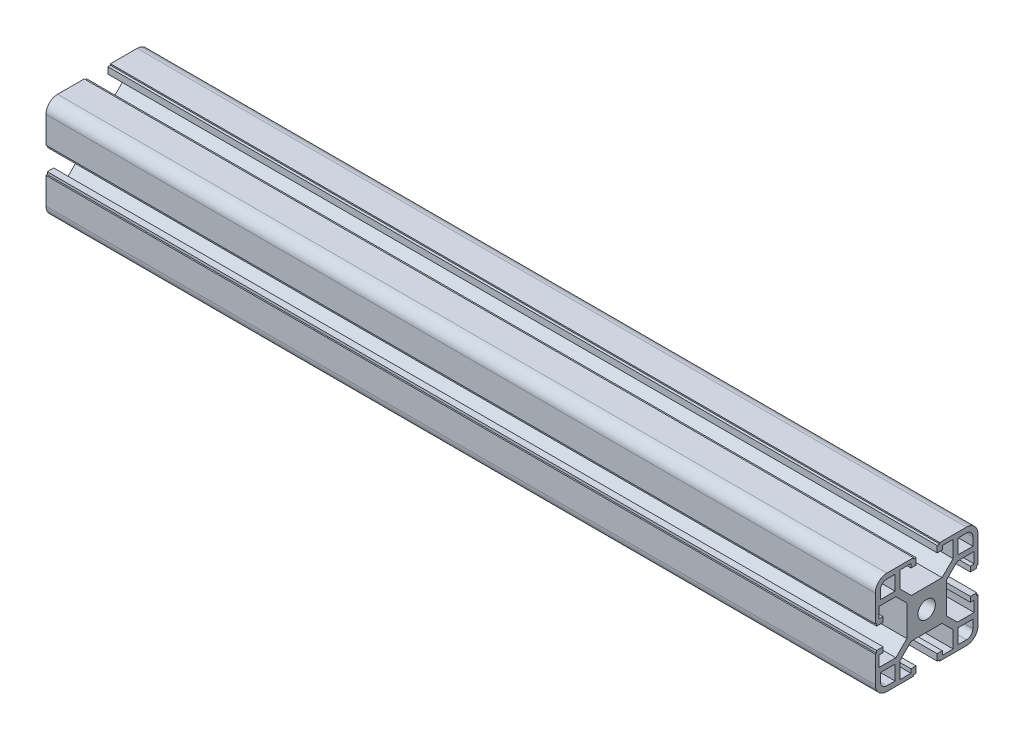
SolidWorks part; units mm, degrees
ref_plane "Front Plane" through (0, 0, 0) normal (0, 0, 1) x (1, 0, 0)
ref_plane "Top Plane" through (0, 0, 0) normal (0, 1, 0) x (1, 0, 0)
ref_plane "Right Plane" through (0, 0, 0) normal (1, 0, 0) x (0, 0, -1)
sketch "草图1" plane through (0, 0, 0) normal (0, 0, 1) x (1, 0, 0)
  line L0 (-984.975, 0) -> (-661.975, 0)
  dimension "D1" = 323
other "Aluminium profile 40 X 40B X R4.5(1)"
ref_plane "Plane1" through (-984.975, 0, 0) normal (1, 0, 0) x (0, 1, 0)
sketch "Sketch1" plane through (-984.975, 0, 0) normal (1, 0, 0) x (0, 1, 0)
  line L0 (-5.1, 20) -> (-5.1, 19.5)
  line L1 (-5.1, 19.5) -> (-4.1, 19.5)
  line L2 (-4.1, 19.5) -> (-4.1, 17)
  line L3 (-6.1, 18.5) -> (-10.3, 18.5)
  line L4 (-15.5, -20) -> (-5.1, -20)
  line L5 (-20, -15.5) -> (-20, -5.1)
  line L6 (15.5, 20) -> (5.1, 20)
  line L7 (20, 15.5) -> (20, 5.1)
  line L8 (0, 14.8756) -> (0, 0) construction
  line L9 (0, 0) -> (14.1675, 0) construction
  line L10 (-10.3, 18.5) -> (-10.3, 12)
  line L11 (-10.3, 12) -> (-6, 7.7)
  line L12 (-6, 7.7) -> (6, 7.7)
  line L13 (10.3, 12) -> (6, 7.7)
  line L14 (10.3, 18.5) -> (10.3, 12)
  line L15 (6.1, 18.5) -> (10.3, 18.5)
  line L16 (4.1, 19.5) -> (4.1, 17)
  line L17 (5.1, 19.5) -> (4.1, 19.5)
  line L18 (5.1, 20) -> (5.1, 19.5)
  line L19 (-5.1, 20) -> (-15.5, 20)
  line L20 (20, 5.1) -> (19.5, 5.1)
  line L21 (12.3, 18) -> (15.5, 18)
  line L22 (12.3, 18) -> (12.3, 12.3)
  line L23 (12.3, 12.3) -> (18, 12.3)
  line L24 (18, 15.5) -> (18, 12.3)
  line L25 (19.5, 5.1) -> (19.5, 4.1)
  line L26 (19.5, 4.1) -> (17, 4.1)
  line L27 (17, 6.1) -> (17, 4.1)
  line L28 (18.5, 6.1) -> (17, 6.1)
  line L29 (18.5, 6.1) -> (18.5, 10.3)
  line L30 (18.5, 10.3) -> (12, 10.3)
  line L31 (12, 10.3) -> (7.7, 6)
  line L32 (7.7, 6) -> (7.7, -6)
  line L33 (12, -10.3) -> (7.7, -6)
  line L34 (18.5, -10.3) -> (12, -10.3)
  line L35 (18.5, -6.1) -> (18.5, -10.3)
  line L36 (18.5, -6.1) -> (17, -6.1)
  line L37 (17, -4.1) -> (17, -6.1)
  line L38 (19.5, -4.1) -> (17, -4.1)
  line L39 (19.5, -5.1) -> (19.5, -4.1)
  line L40 (20, -5.1) -> (19.5, -5.1)
  line L41 (5.1, -20) -> (5.1, -19.5)
  line L42 (5.1, -19.5) -> (4.1, -19.5)
  line L43 (4.1, -19.5) -> (4.1, -17)
  line L44 (6.1, -17) -> (4.1, -17)
  line L45 (6.1, -18.5) -> (6.1, -17)
  line L46 (6.1, -18.5) -> (10.3, -18.5)
  line L47 (10.3, -18.5) -> (10.3, -12)
  line L48 (10.3, -12) -> (6, -7.7)
  line L49 (6, -7.7) -> (-6, -7.7)
  line L50 (-10.3, -12) -> (-6, -7.7)
  line L51 (-10.3, -18.5) -> (-10.3, -12)
  line L52 (-6.1, -18.5) -> (-10.3, -18.5)
  line L53 (-6.1, -18.5) -> (-6.1, -17)
  line L54 (-4.1, -17) -> (-6.1, -17)
  line L55 (-4.1, -19.5) -> (-4.1, -17)
  line L56 (-5.1, -19.5) -> (-4.1, -19.5)
  line L57 (-5.1, -20) -> (-5.1, -19.5)
  line L58 (-20, -5.1) -> (-19.5, -5.1)
  line L59 (5.1, -20) -> (15.5, -20)
  line L60 (-20, 5.1) -> (-20, 15.5)
  line L61 (-19.5, -5.1) -> (-19.5, -4.1)
  line L62 (-6.1, 18.5) -> (-6.1, 17)
  line L63 (-6.1, 17) -> (-4.1, 17)
  line L64 (6.1, 18.5) -> (6.1, 17)
  line L65 (4.1, 17) -> (6.1, 17)
  line L66 (-19.5, -4.1) -> (-17, -4.1)
  line L67 (-15.5, 18) -> (-12.3, 18)
  line L68 (-18, 15.5) -> (-18, 12.3)
  line L69 (-18, 12.3) -> (-12.3, 12.3)
  line L70 (-12.3, 18) -> (-12.3, 12.3)
  line L71 (-17, -6.1) -> (-17, -4.1)
  line L72 (-18.5, -6.1) -> (-17, -6.1)
  line L73 (-18.5, -6.1) -> (-18.5, -10.3)
  line L74 (-18.5, -10.3) -> (-12, -10.3)
  line L75 (-12, -10.3) -> (-7.7, -6)
  line L76 (-7.7, -6) -> (-7.7, 6)
  line L77 (-12, 10.3) -> (-7.7, 6)
  line L78 (-18.5, 10.3) -> (-12, 10.3)
  line L79 (-18.5, 6.1) -> (-18.5, 10.3)
  line L80 (-18.5, 6.1) -> (-17, 6.1)
  line L81 (-17, 4.1) -> (-17, 6.1)
  line L82 (-19.5, 4.1) -> (-17, 4.1)
  line L83 (-19.5, 5.1) -> (-19.5, 4.1)
  line L84 (-20, 5.1) -> (-19.5, 5.1)
  line L85 (20, -5.1) -> (20, -15.5)
  line L87 (-18, -12.3) -> (-12.3, -12.3)
  line L88 (-18, -12.3) -> (-18, -15.5)
  line L89 (-15.5, -18) -> (-12.3, -18)
  line L90 (-12.3, -12.3) -> (-12.3, -18)
  line L91 (12.3, -12.3) -> (18, -12.3)
  line L92 (12.3, -12.3) -> (12.3, -18)
  line L93 (12.3, -18) -> (15.5, -18)
  line L94 (18, -12.3) -> (18, -15.5)
  circle A0 centre (0, 0) radius 3.4
  arc A1 (-20, 15.5) -> (-15.5, 20) centre (-15.5, 15.5) cw
  arc A2 (20, 15.5) -> (15.5, 20) centre (15.5, 15.5) ccw
  arc A3 (-15.5, -20) -> (-20, -15.5) centre (-15.5, -15.5) cw
  arc A4 (15.5, -20) -> (20, -15.5) centre (15.5, -15.5) ccw
  arc A5 (-15.5, 18) -> (-18, 15.5) centre (-15.5, 15.5) ccw
  arc A6 (18, 15.5) -> (15.5, 18) centre (15.5, 15.5) ccw
  arc A7 (18, -15.5) -> (15.5, -18) centre (15.5, -15.5) cw
  arc A8 (-18, -15.5) -> (-15.5, -18) centre (-15.5, -15.5) ccw
  point P2 (0, 10)
  point P4 (0, 0)
  point P5 (-20, -20)
  point P6 (20, -20)
  point P7 (20, 20)
  point P8 (-20, 20)
  point P36 (-20, 20)
  point P39 (20, 20)
  point P121 (0, 0)
  dimension "D1" = 20.6
  dimension "D2" = 40
  dimension "D3" = 8.2
  dimension "D4" = 10.2
  dimension "D5" = 12.3
  dimension "D6" = 6.8
  dimension "D7" = 4.5
  dimension "D8" = 45
  dimension "D12" = 2
  dimension "D13" = 5.7
  dimension "D14" = 2
  dimension "D18" = 2.5
  dimension "D19" = 2.5
  dimension "D15" = 2.5
  dimension "D9" = 0.5
  dimension "D10" = 1.5
  dimension "D11" = 12
  dimension "D16" = 3
  dimension "D17" = 2
  dimension "D20" = 2
  dimension "D21" = 2
